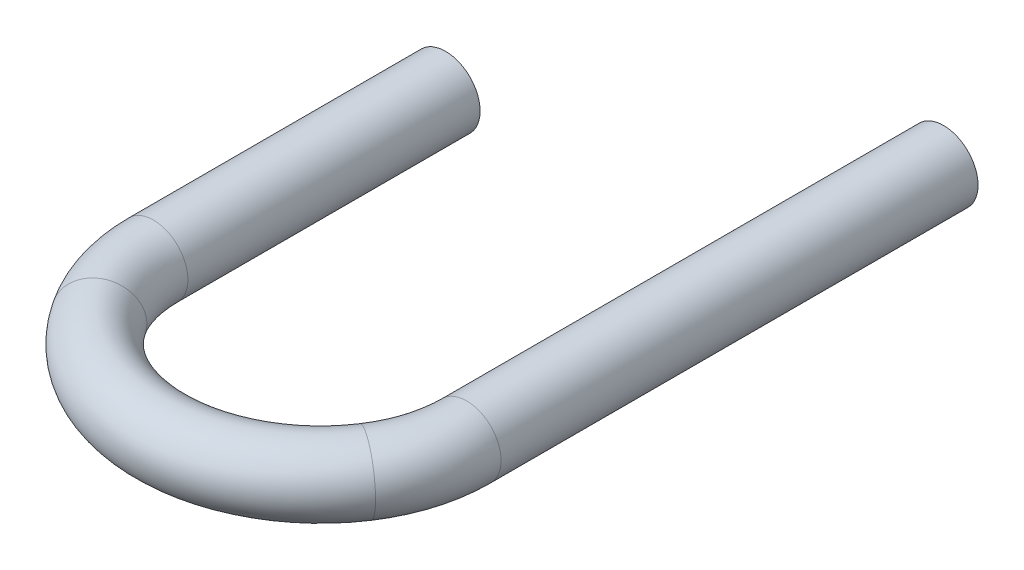
from build123d import *

# Parameters (mm, degrees)
SKETCH1_R   = 11
SKETCH1_R_2 = 7.5


with BuildPart() as part:
    # Sweep1: sweep along a path in Sketch2
    with BuildLine(Plane(origin=(0, 0, 0), x_dir=(1, 0, 0), z_dir=(0, 1, 0))) as sweep1_path:
        Line((0, 0), (0, -93.298854008))
        ThreePointArc((0, -93.298854008), (1.899755617, -106.235968606), (7.438619295, -118.080756266))
        ThreePointArc((7.438619295, -118.080756266), (50, -140.990195136), (92.561380705, -118.080756266))
        ThreePointArc((92.561380705, -118.080756266), (98.100244383, -106.235968606), (100, -93.298854008))
        Line((100, -93.298854008), (100, 59.000000002))
    # Sketch1 → Sweep1 (sweep)
    with BuildSketch(Plane.XY):
        Circle(SKETCH1_R)
        Circle(SKETCH1_R_2, mode=Mode.SUBTRACT)
    sweep(path=sweep1_path.line)


solid = part.part
